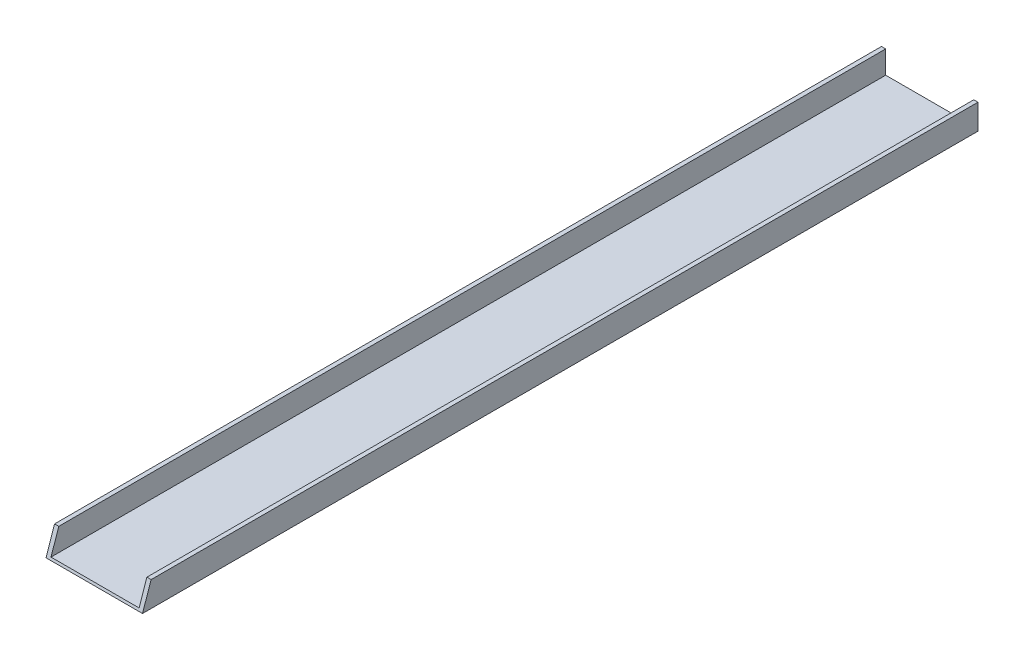
from build123d import *

# Parameters (mm, degrees)
BOSS_EXTRUDE1_DEPTH = 1099.3375
CUT_EXTRUDE1_DEPTH  = 150


with BuildPart() as part:
    # Sketch1 → Boss-Extrude1 (new, symmetric)
    with BuildSketch(Plane.XY):
        Polygon((127, 0), (-127, 0), (-127, 66.04), (-115.9256, 66.04), (-115.9256, 6.096), (115.9256, 6.096), (115.9256, 66.04), (127, 66.04), align=None)
    extrude(amount=BOSS_EXTRUDE1_DEPTH, both=True)

    # Sketch2 → Cut-Extrude1 (cut, symmetric)
    with BuildSketch(Plane(origin=(0, 0, 0), x_dir=(0, 0, -1), z_dir=(1, 0, 0))):
        Polygon((-1099.3375, 0), (-1076.752705704, 66.04), (-1099.3375, 66.04), align=None)
    extrude(amount=CUT_EXTRUDE1_DEPTH, both=True, mode=Mode.SUBTRACT)


solid = part.part
